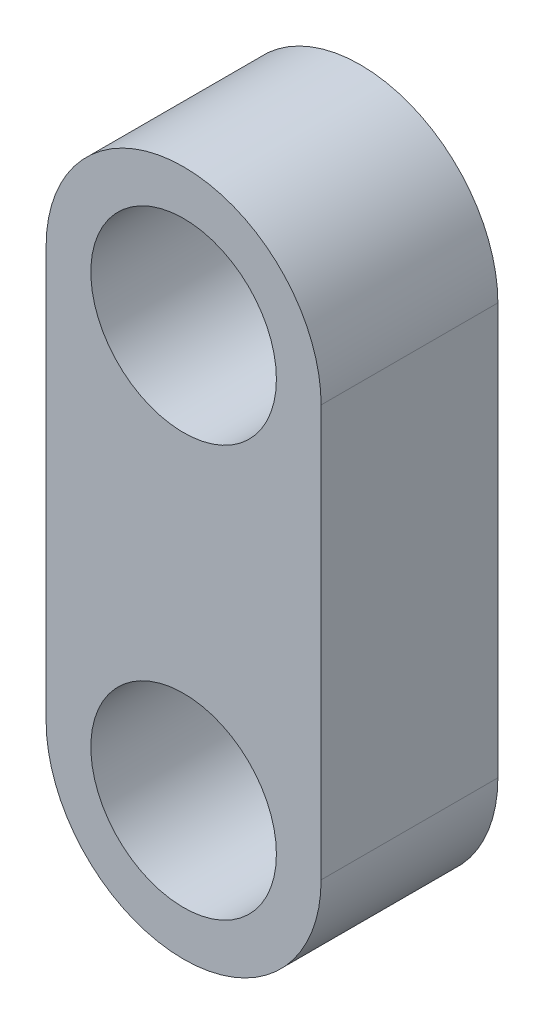
from build123d import *

# Parameters (mm, degrees)
BOSS_EXTRUDE2_DEPTH = 3.5
SKETCH4_R           = 3.674588618
CUT_EXTRUDE1_DEPTH  = 10
SKETCH2_R           = 3.674588618
CUT_EXTRUDE2_DEPTH  = 10


with BuildPart() as part:
    # Sketch1 → Boss-Extrude2 (new, symmetric)
    with BuildSketch(Plane.XY):
        with BuildLine():
            Line((-32.510632707, 16.288746435), (-32.510632707, 0))
            ThreePointArc((-32.510632707, 0), (-27.065651732, -5.444980975), (-21.620670757, 0))
            Line((-21.620670757, 0), (-21.620670757, 16.288746435))
            ThreePointArc((-21.620670757, 16.288746435), (-27.065651732, 21.73372741), (-32.510632707, 16.288746435))
        make_face()
    extrude(amount=BOSS_EXTRUDE2_DEPTH, both=True)

    # Sketch4 → Cut-Extrude1 (cut)
    with BuildSketch(Plane.XY.offset(3.5)):
        with Locations((-27.065651732, 0)):
            Circle(SKETCH4_R)
    extrude(amount=-CUT_EXTRUDE1_DEPTH, mode=Mode.SUBTRACT)

    # Sketch2 → Cut-Extrude2 (cut)
    with BuildSketch(Plane.XY.offset(3.5)):
        with Locations((-27.065651732, 16.288746435)):
            Circle(SKETCH2_R)
    extrude(amount=-CUT_EXTRUDE2_DEPTH, mode=Mode.SUBTRACT)


solid = part.part
